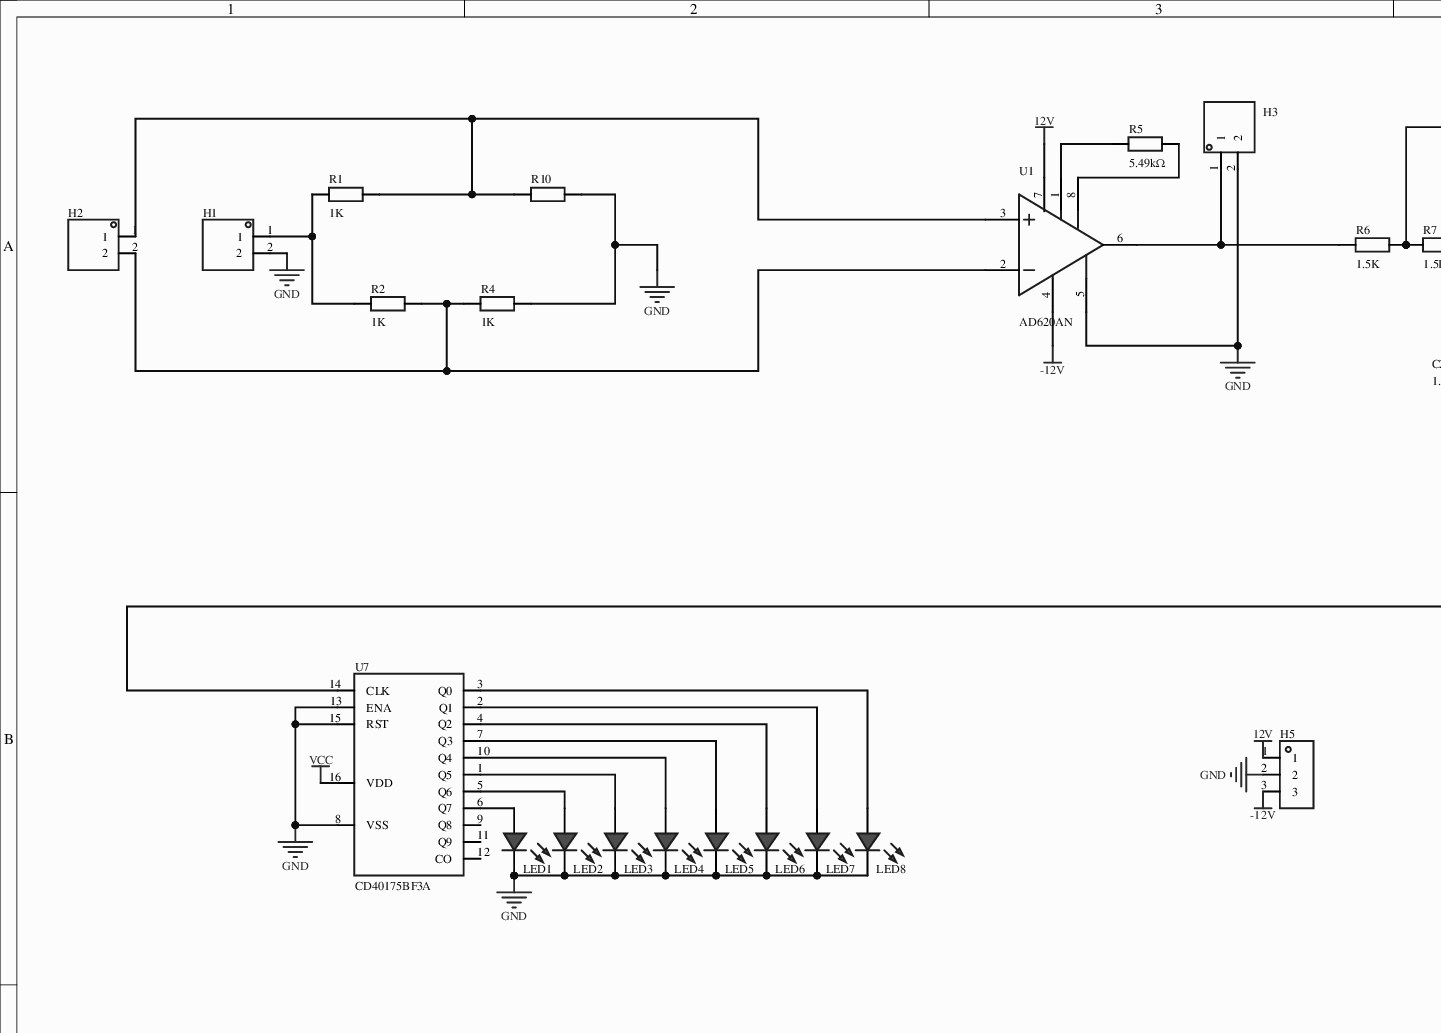
[diagram p0: MISC51786-3.schdoc, top left]
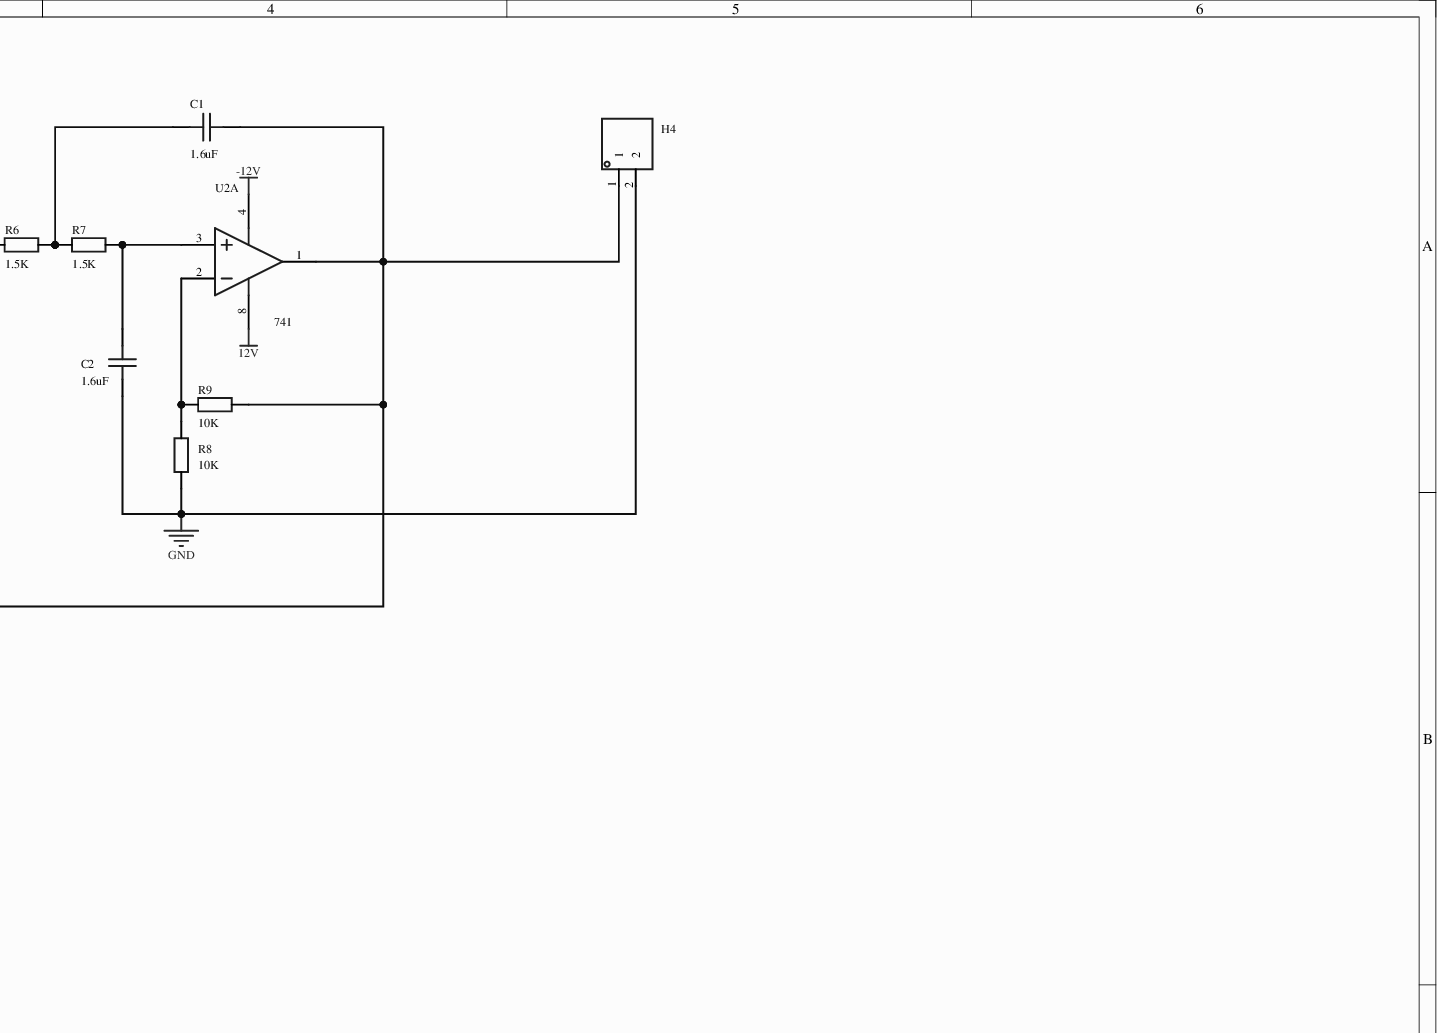
[diagram p1: MISC51786-3.schdoc, top right]
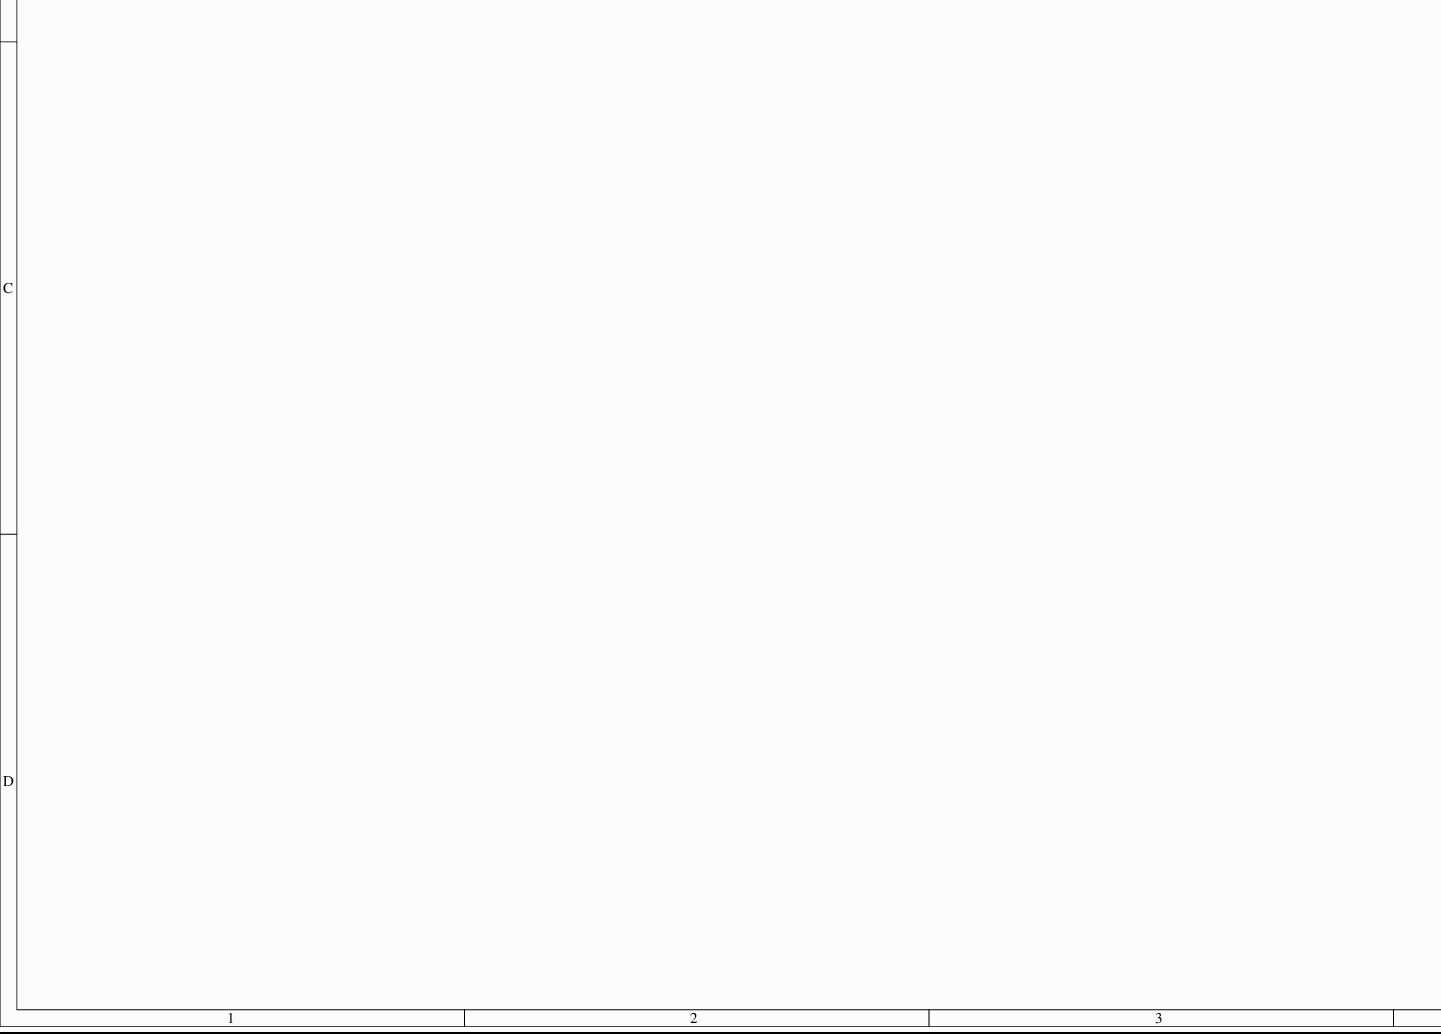
[diagram p2: MISC51786-3.schdoc, bottom left]
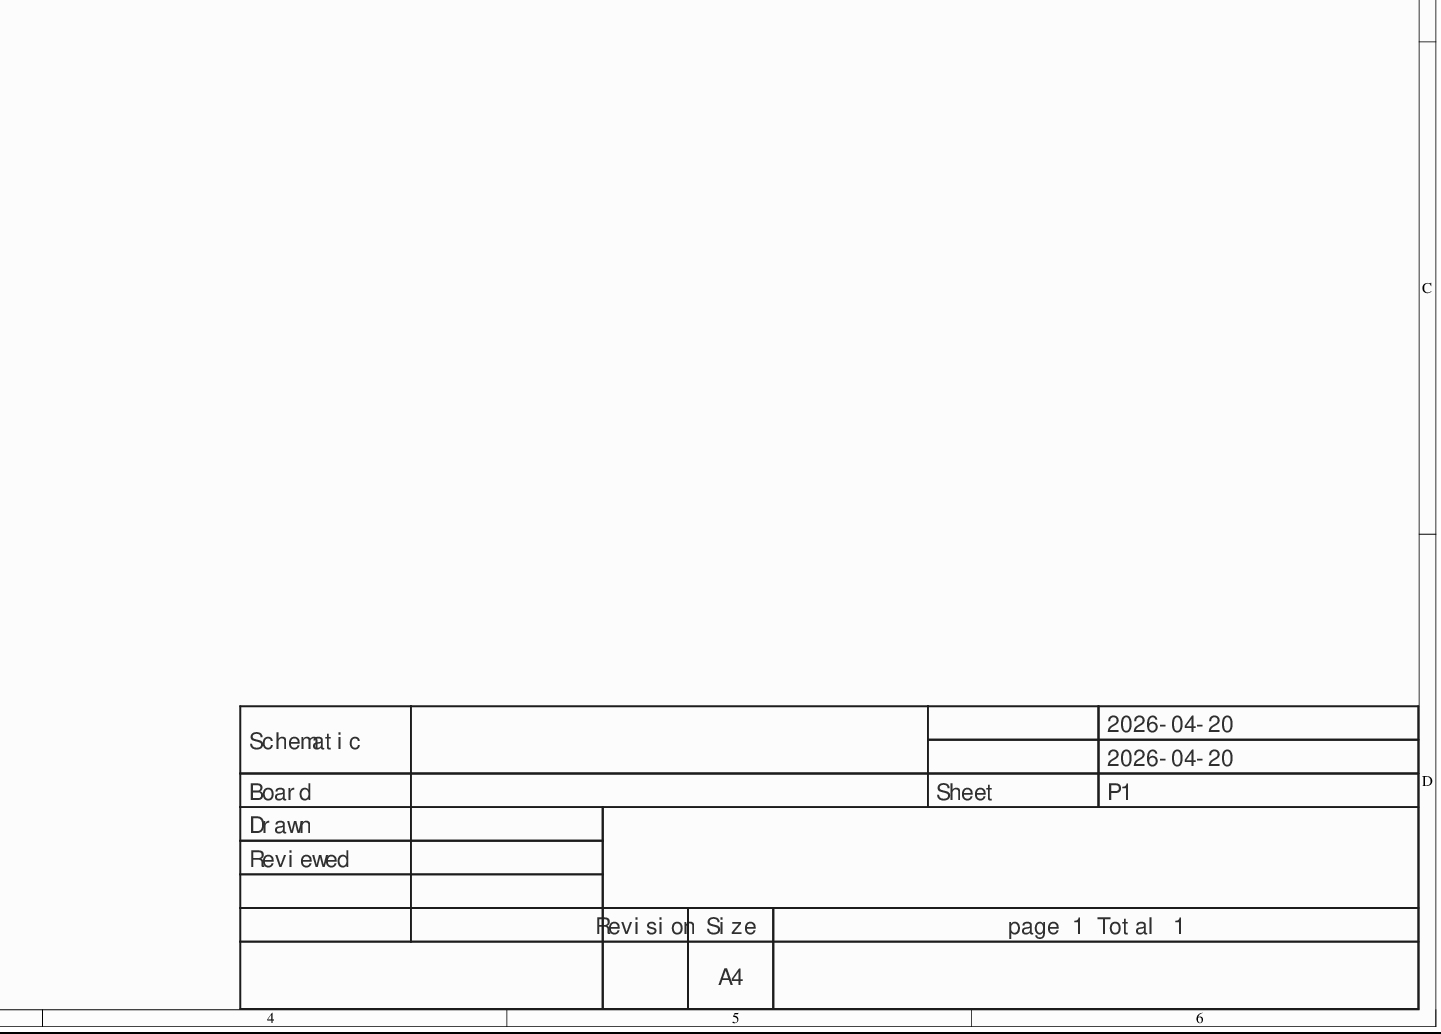
[diagram p3: MISC51786-3.schdoc, bottom right]
# Altium project MISC51786-2.PrjPcb
1 sheet, 27 parts. Net scope: global (net labels, ports and power ports of the same name join across sheets).
Board file: MISC51786.pcbdoc

## Sheet MISC51786-3.schdoc
size 420 x 297 mm; Version: V1.0; @Project Name: MISC51786; @Update Date: 2026-04-20; @Create Date: 2026-04-20; @Board Name: MISC51786; @Create Time: 00:26:06; @Page Count: 1; @Page No: 1; @Schematic Name: MISC51786; @Update Time: 00:26:06; Size: A4

### Parts
C1  1.6uF  [C0603]
C2  1.6uF  [C0603]
H1  (no value)  [HDR-TH_2P-P2.54-V-M-1]
H2  (no value)  [HDR-TH_2P-P2.54-V-M-1]
H3  (no value)  [HDR-TH_2P-P2.54-V-M-1]
H4  (no value)  [HDR-TH_2P-P2.54-V-M-1]
H5  (no value)  [HDR-TH_3P-P2.54-V-F]
LED1  (no value)  [LED_TH-3mm]
LED2  (no value)  [LED_TH-3mm]
LED3  (no value)  [LED_TH-3mm]
LED4  (no value)  [LED_TH-3mm]
LED5  (no value)  [LED_TH-3mm]
LED6  (no value)  [LED_TH-3mm]
LED7  (no value)  [LED_TH-3mm]
LED8  (no value)  [LED_TH-3mm]
R1  1K  [R0603]
R2  1K  [R0603]
R4  1K  [R0603]
R5  5.49kΩ  [R0603]
R6  1.5K  [R0603]
R7  1.5K  [R0603]
R8  10K  [R0603]
R9  10K  [R0603]
R10  10kΩ  [Res_1/8W]  (value not drawn)
U1  AD620AN  [DIP-8_L9.3-W6.4-P2.54-LS7.6-BL]
U2  741  [PDIP-8_L10.2-W6.5-P2.54-LS7.6-BL]  (part A of 2)
U7  CD40175BF3A  [CDIP-16_L21.4-W6.8-P2.54-LS7.8-BL]

### Nets
12V: H5.1 U1.7(+VS) U2.8(V+)
-12V: H5.3 U1.4(-VS) U2.4(GND)
GND: C2.1 H1.2 H3.2 H4.2 H5.2 LED1.2(A) LED2.2(A) LED3.2(A) LED4.2(A) LED5.2(A) LED6.2(A) LED7.2(A) LED8.2(A) R4.2 R8.1 R10.2 U1.5(REF) U7.8(VSS) U7.13(ENA) U7.15(RST)
VCC: U7.16(VDD)
NetC1_1: C1.1 R6.1 R7.2
NetC1_2: C1.2 H4.1 R9.1 U2.1(OUTA) U7.14(CLK)
NetC2_2: C2.2 R7.1 U2.3(INA+)
NetH1_1: H1.1 R1.1 R2.1
NetH2_1: H2.1 R1.2 R10.1 U1.3(+IN)
NetH2_2: H2.2 R2.2 R4.1 U1.2(-IN)
NetH3_1: H3.1 R6.2 U1.6(OUTPUT)
NetLED1_1: LED1.1(C) U7.6(Q7)
NetLED2_1: LED2.1(C) U7.5(Q6)
NetLED3_1: LED3.1(C) U7.1(Q5)
NetLED4_1: LED4.1(C) U7.10(Q4)
NetLED5_1: LED5.1(C) U7.7(Q3)
NetLED6_1: LED6.1(C) U7.4(Q2)
NetLED7_1: LED7.1(C) U7.2(Q1)
NetLED8_1: LED8.1(C) U7.3(Q0)
NetR5_1: R5.1 U1.1(RG)
NetR5_2: R5.2 U1.8(RG)
NetR8_2: R8.2 R9.2 U2.2(INA-)

Not connected (* = marked no-connect by the designer): U7 9(Q8) 11(Q9) 12(CO)

### Notes on the sheet
- 2026-04-20
- Schematic
- Board
- Sheet
- P1
- Drawn
- Reviewed
- Revision
- Size
- A4
- page 1 Total 1

### Library data of the parts
C1 C2 = CAP_0603: Symbol: Capacitance; ConvertToPcb: yes; ModelId: ac125912035d415993ca9572d50418b10819f05c4eef4c71ace90d822a990e87; ModelName: C0603_L1.6-W0.8-H0.8; ModelTransform: 62.992,31.496,0,0,0,0,0,0,0; Device: CAP_0603; Value: 1.6uF; AddInBom: yes; Supplier Footprint: 0603; FootprintName: C0603
H1-H4 = HDR-M_2.54_1x2P: Symbol: 210S-1*2P L=11.6MMGold-plated black; ConvertToPcb: yes; ModelId: 79b2e9f2d70a4d68a1b7098f27c6d4c50819f05c4eef4c71ace90d822a990e87; ModelName: HDR-M-2.54_1x2; ModelTransform: 200,100,0,0,0,0,0,0,-118.11; Device: HDR-M_2.54_1x2P; AddInBom: yes; SupplierPart: C124375; Supplier Footprint: 插件; FootprintName: HDR-TH_2P-P2.54-V-M-1
H5 = HDR-F_2.54_1x3P: Symbol: PM254V-11-03-H85; ConvertToPcb: yes; ModelId: f3b3cc5aae9641bf9e56fc160cef875b0819f05c4eef4c71ace90d822a990e87; ModelName: HDR2.54-F-LI-1X3P; ModelTransform: 299.9994,100,0,0,0,0,0,0,-118.11; Device: HDR-F_2.54_1x3P; AddInBom: yes; SupplierPart: C541850; Supplier Footprint: 插件; FootprintName: HDR-TH_3P-P2.54-V-F
LED1-LED8 = LED_TH-R_3mm: ConvertToPcb: yes; ModelId: a497c992633541038a38947cdc58012f0819f05c4eef4c71ace90d822a990e87; ModelName: LED-TH-3mm_R; ModelTransform: 141.274,153.327,0,0,0,0,-5.984,0,-137.795; Symbol: LED_TH-R; Device: LED_TH-R_3mm; AddInBom: yes; FootprintName: LED_TH-3mm; Supplier Footprint: 插件
R1 R2 R4-R9 = Res_0603: Symbol: Resistor; ConvertToPcb: yes; ModelId: fc143cca1e79419f9cd78b61e9279f080819f05c4eef4c71ace90d822a990e87; ModelTransform: 31.8897,63.7794,0,90,0,0,0,0,0; Device: Res_0603; AddInBom: yes; Supplier Footprint: 0603; FootprintName: R0603; ModelName: R0603
  R1 R2 R4: Value: 1K
  R5: Value: 5.49kΩ
  R6 R7: Value: 1.5K
  R8 R9: Value: 10K
R10 = Res_AXIAL-1/8W: Symbol: Resistor; 3D Model: b2b5ae7ae4c642178fe0039925c86a3f0819f05c4eef4c71ace90d822a990e87; 3D Model Transform: 282.86,66.88,253.09,0,0,0,0,0,-191; ConvertToPcb: yes; ModelName: RES-TH_BD1.8-L3.2-P7.20-D0.4; Device: Res_AXIAL-1/8W; Supplier Footprint: 轴向引线; Value: 10kΩ; AddInBom: yes; FootprintName: Res_1/8W
U1 = AD620ANZ: Amplifier count: single; CMRR: 100dB; input bias current (Ib): 500pA; input offset voltage (Vos): 30uV; gain-bandwidth product (GBP): -; slew rate (SR): 0.75V/us; bandwidth (-3dB): 120kHz;; Manufacturer: ADI(亚德诺); Symbol: AD620ANZ_1; AddInBom: yes; ModelId: e1ba2ac1384341a197ae27979c8d89420819f05c4eef4c71ace90d822a990e87; ModelName: DIP-8_L9.3-W6.4-H4.5-P2.54-LS7.6-BL; ModelTransform: 364.173,311.8104,0,0,0,0,0,0,-118.11; Voltage - Supply: 2.3V~18V; -18V~-2.3V; Output Current: 18mA; Quiescent Current per Amplifier: 1.3mA; Input Offset Voltage Drift(Vos TC): 0.3uV/℃; Device: AD620ANZ; Manufacturer Part: AD620AN; LCSC Part Name: 低成本低功耗仪表放大器; SupplierPart: C9680; Supplier Footprint: DIP-8; JLCPCB Part Class: Extended Part; Datasheet: example.com/datasheet/AD620ANZ/10210.html; Supplier: LCSC; ConvertToPcb: yes; FootprintName: DIP-8_L9.3-W6.4-P2.54-LS7.6-BL; Number of Channels: Single; Common Mode Rejection Ratio(CMRR): 100dB; Ib - Input Bias Current: 500pA; Vos - Input Offset Voltage: 30uV; Gain Bandwidth Product: -; Slew Rate: 0.75V/us; -3dB Bandwidth: 120kHz; Operating Temperature: -40℃~+85℃
U2 = LM358AN/NOPB: Amplifier count: 2; rail-to-rail: -; gain-bandwidth product (GBW): 1MHz; input offset voltage (Vos): 2mV; slew rate (SR): -; input bias current (Ib): 50nA;; Manufacturer: TI(德州仪器); Relevance: []; AddInBom: yes; ModelId: b5bb019b7dad497cba3f645155e53c260819f05c4eef4c71ace90d822a990e87; ModelTransform: 401.574,311.8104,0,0,0,0,0,0,-137.795; Number of Channels: 2; Maximum Power Supply Range (Vdd-Vss): 32V; Input Offset Voltage Drift(Vos TC): 7uV/℃; Common Mode Rejection Ratio(CMRR): 85dB; Quiescent Current: 500uA; Output Current: 40mA; Single supply: 3V~32V; Dual Supply: -16V~-1.5V; 1.5V~16V; Symbol: LM358AN/NOPB; Device: LM358AN/NOPB; Manufacturer Part: 741; LCSC Part Name: LM358AN/NOPB; SupplierPart: C1348620; Supplier Footprint: PDIP-8; JLCPCB Part Class: Extended Part; Supplier: LCSC; ConvertToPcb: yes; FootprintName: PDIP-8_L10.2-W6.5-P2.54-LS7.6-BL; ModelName: PDIP-8_L10.2-W6.5-P2.54-LS7.6-BL; Rail to Rail: -; Gain Bandwidth Product: 1MHz; Vos - Input Offset Voltage: 2mV; Slew Rate: -; Ib - Input Bias Current: 50nA; Input Offset Current(Ios): 50nA; Input Voltage Noise Density: -; Input offset current drift(Ios TC): -; Operating Temperature: 0℃~+70℃
U7 = CD40175BF3A: CD40175B-MIL CMOS quad D-type flip-flop; Manufacturer: TI(德州仪器); 3D Model: a910f5494e794b9ab944fba836aa86d50819f05c4eef4c71ace90d822a990e87; 3D Model Transform: 787.4,311.8104,0,0,0,0,0,0,-118.11; AddInBom: yes; ModelName: CDIP-16_L21.4-W6.8-H5.1-P2.54-LS7.8-BL; Symbol: CD40175BF3A; Device: CD40175BF3A; LCSC Part Name: CD40175BF3A; Supplier Part: C3826078; Manufacturer Part: CD40175BF3A; Supplier Footprint: CDIP-16; JLCPCB Part Class: Extended Part; Supplier: LCSC; ConvertToPcb: yes; FootprintName: CDIP-16_L21.4-W6.8-P2.54-LS7.8-BL